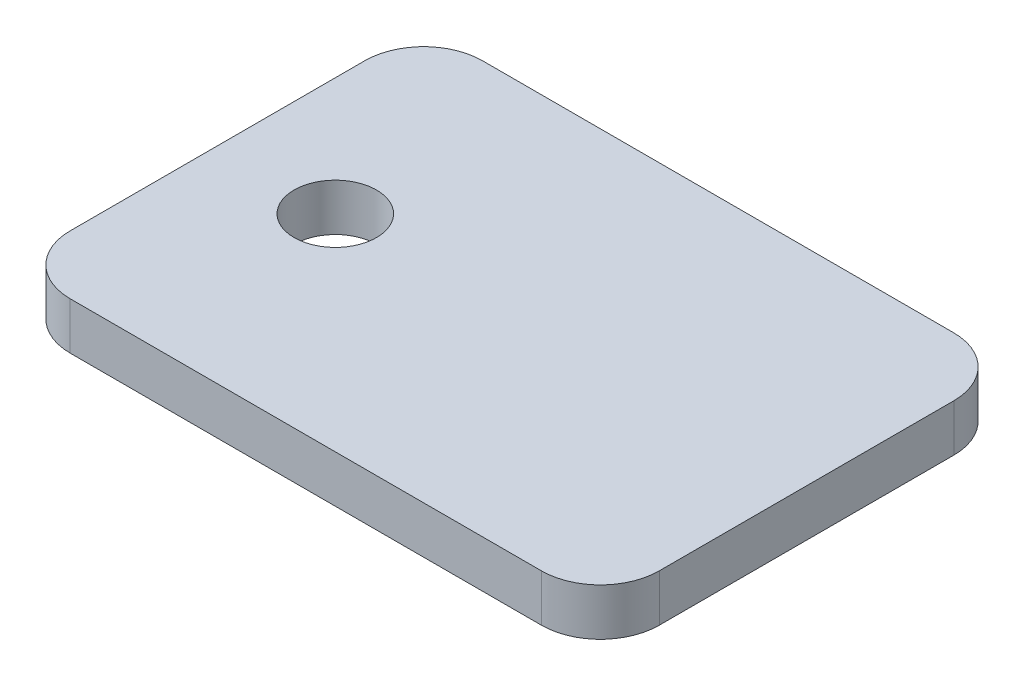
from build123d import *

# Parameters (mm, degrees)
SKETCH1_W           = 100
SKETCH1_H           = 70
BOSS_EXTRUDE1_DEPTH = 8
FILLET1_R           = 10
SKETCH2_R           = 7
CUT_EXTRUDE1_DEPTH  = 8


with BuildPart() as part:
    # Sketch1 → Boss-Extrude1 (new body)
    with BuildSketch(Plane(origin=(0, 0, 0), x_dir=(1, 0, 0), z_dir=(0, 1, 0))):
        Rectangle(SKETCH1_W, SKETCH1_H)
    extrude(amount=BOSS_EXTRUDE1_DEPTH)

    # Fillet1
    fillet1_edges = [part.edges().sort_by_distance(p)[0] for p in [
        (-50, 4, -35),
        (50, 4, -35),
        (50, 4, 35),
        (-50, 4, 35),
    ]]
    fillet(fillet1_edges, radius=FILLET1_R)

    # Sketch2 → Cut-Extrude1 (cut)
    with BuildSketch(Plane(origin=(0, 8, 0), x_dir=(1, 0, 0), z_dir=(0, 1, 0))):
        with Locations(Location((-30, 0, 0), (0, 0, 270))):
            Circle(SKETCH2_R)
    extrude(amount=-CUT_EXTRUDE1_DEPTH, mode=Mode.SUBTRACT)


solid = part.part
